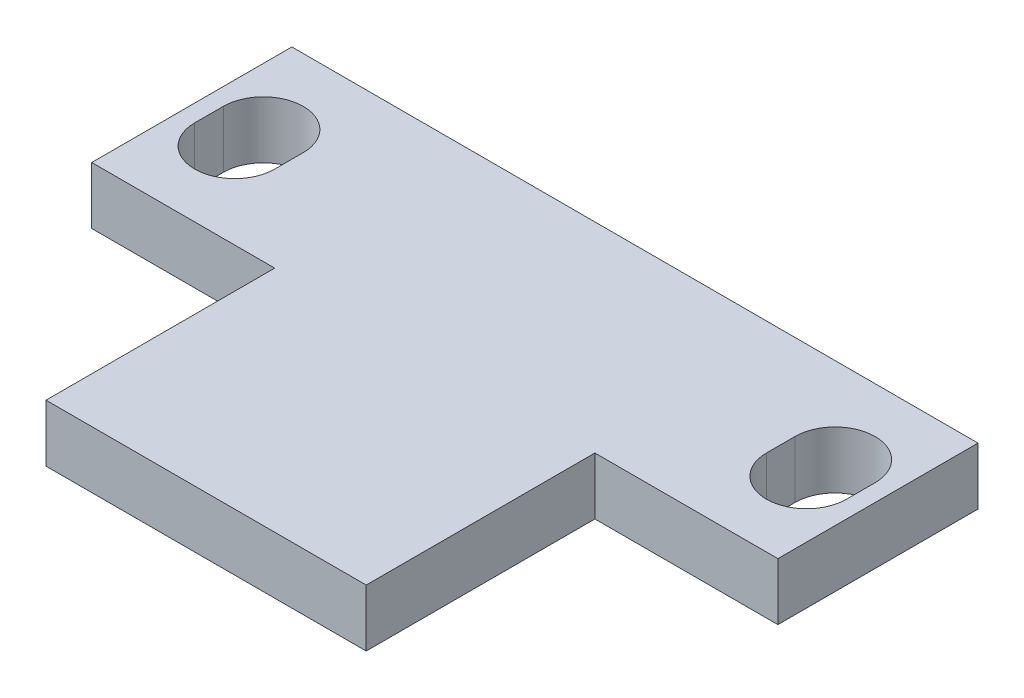
SolidWorks part; units mm, degrees
material "Q235B"
ref_plane "Front Plane" through (0, 0, 0) normal (0, 0, 1) x (1, 0, 0)
ref_plane "Top Plane" through (0, 0, 0) normal (0, 1, 0) x (1, 0, 0)
ref_plane "Right Plane" through (0, 0, 0) normal (1, 0, 0) x (0, 0, -1)
other "Configuration Table"
sketch "Sketch1" plane through (0, 0, 0) normal (0, 1, 0) x (1, 0, 0)
  line L0 (-60, 2.5) -> (-28, 2.5)
  line L1 (-60, -37.5) -> (60, -37.5)
  line L2 (-60, -37.5) -> (-60, 37.5)
  line L3 (-60, 37.5) -> (60, 37.5)
  line L4 (60, -37.5) -> (60, 37.5)
  line L5 (-60, -37.5) -> (60, 37.5) construction
  line L6 (-60, 37.5) -> (60, -37.5) construction
  line L7 (-28, 2.5) -> (-28, -37.5)
  line L8 (28, -37.5) -> (28, 2.5)
  line L9 (28, 2.5) -> (60, 2.5)
  line L10 (-50, 22.5) -> (-50, 17.5) construction
  line L11 (-43, 22.5) -> (-43, 17.5)
  line L12 (-57, 22.5) -> (-57, 17.5)
  line L13 (0, 0) -> (0, 17.5) construction
  line L14 (50, 22.5) -> (50, 17.5) construction
  line L15 (43, 22.5) -> (43, 17.5)
  line L16 (57, 22.5) -> (57, 17.5)
  arc A0 (-43, 22.5) -> (-57, 22.5) centre (-50, 22.5) ccw
  arc A1 (-57, 17.5) -> (-43, 17.5) centre (-50, 17.5) ccw
  arc A2 (43, 22.5) -> (57, 22.5) centre (50, 22.5) cw
  arc A3 (57, 17.5) -> (43, 17.5) centre (50, 17.5) cw
  point P0 (0, 0)
  point P14 (-50, 20)
  point P19 (-50, 29.5)
  point P20 (-50, 10.5)
  point P25 (50, 20)
  dimension "D9" = 7
  dimension "D1" = 120
  dimension "D2" = 75
  dimension "D3" = 56
  dimension "D4" = 28
  dimension "D5" = 35
  dimension "D6" = 35
  dimension "D7" = 19
  dimension "D8" = 10
  dimension "D10" = 17.5
extrude "Boss-Extrude1" add sketch "Sketch1" along normal blind 10 contours L8 L9 L4 L3 L2 L0 L7 L1 A1 L12 A0 L11 L16 A3 L15 A2
